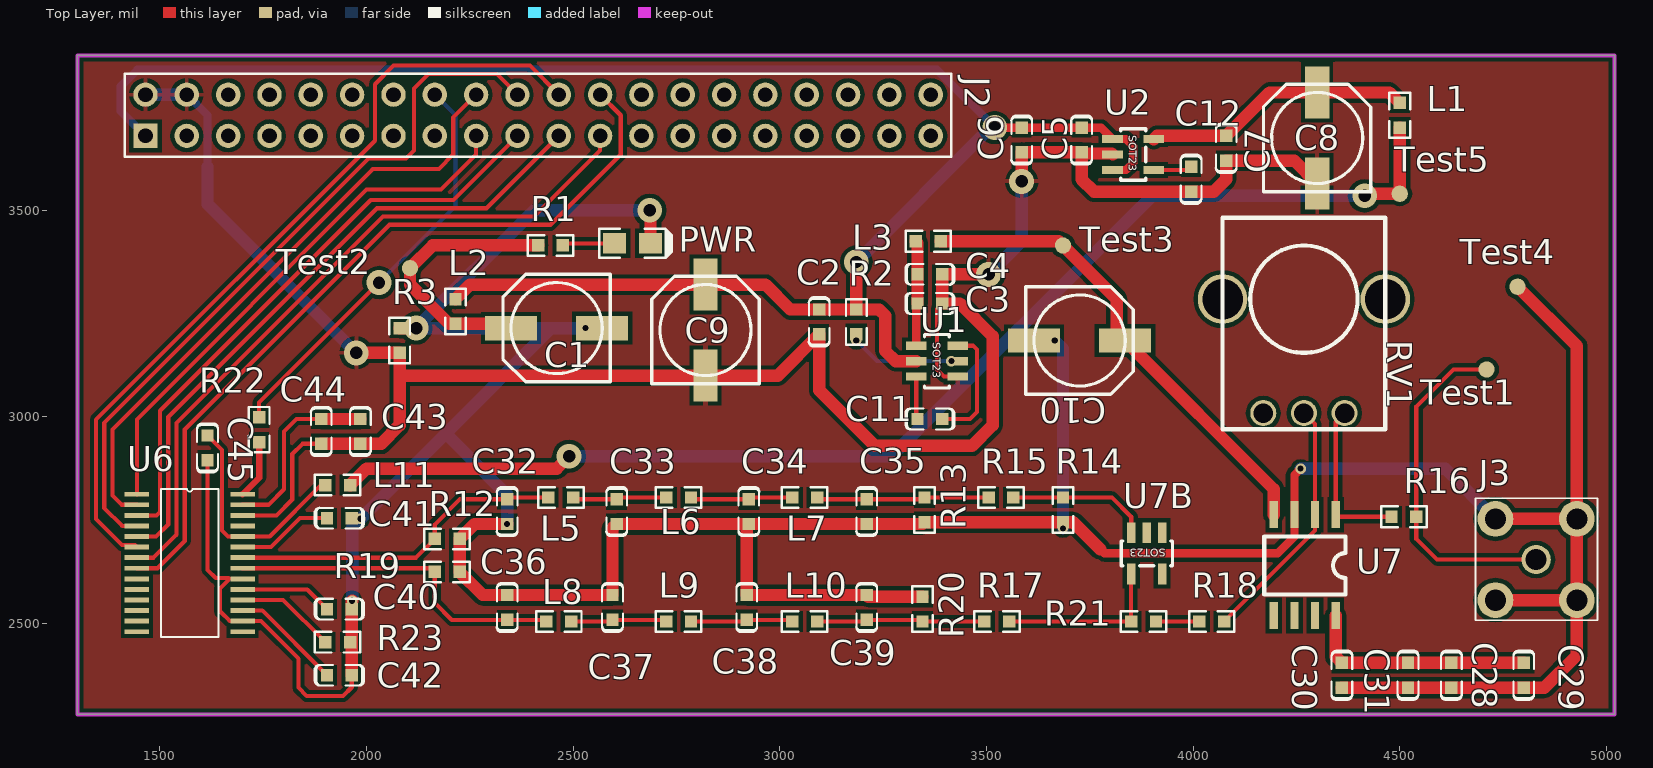
[diagram p0: Top Layer view]
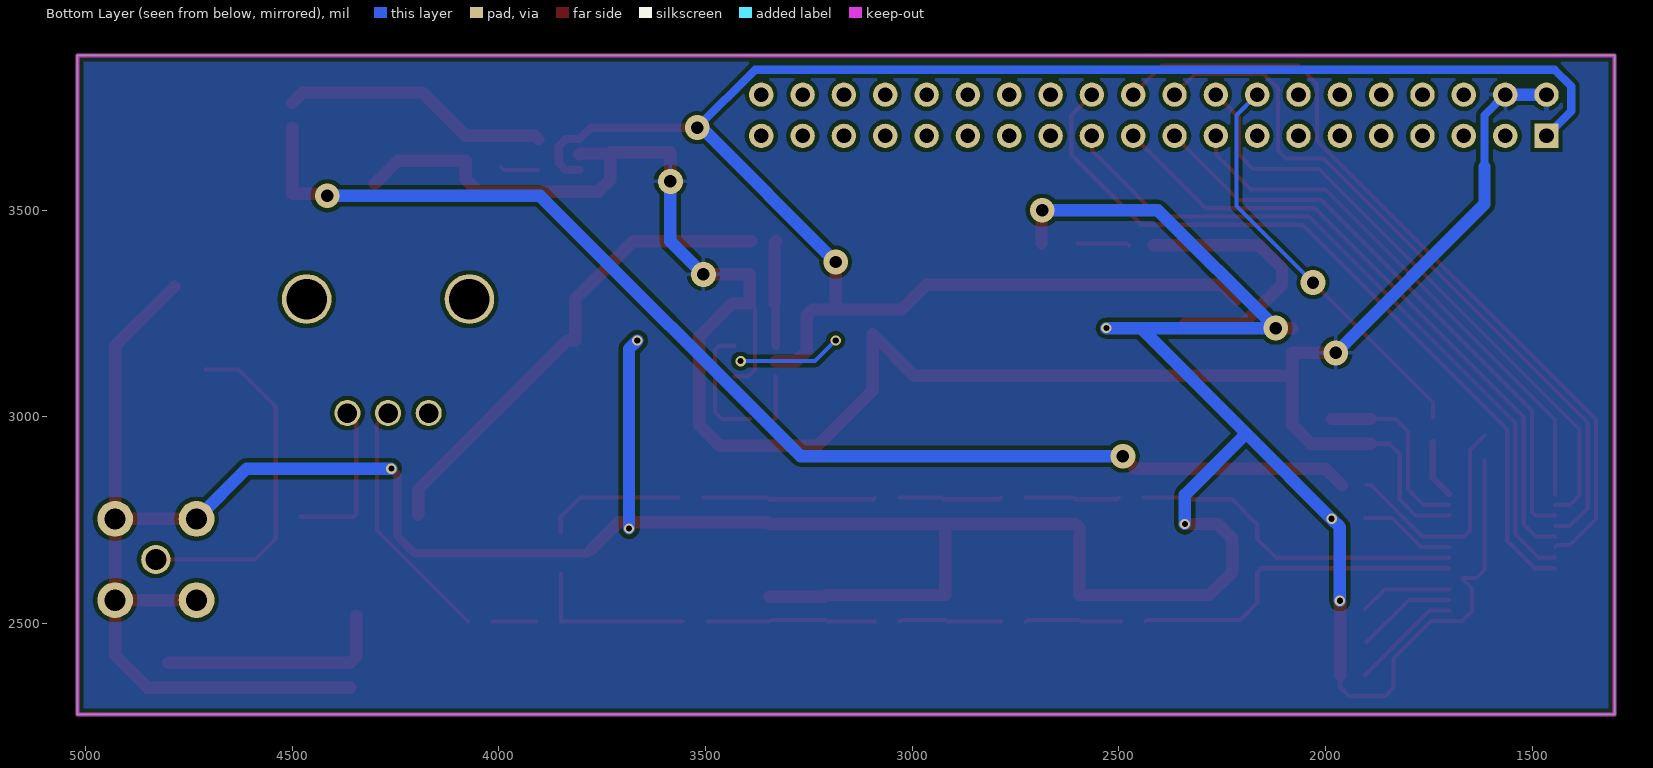
[diagram p1: Bottom Layer view, seen from below]
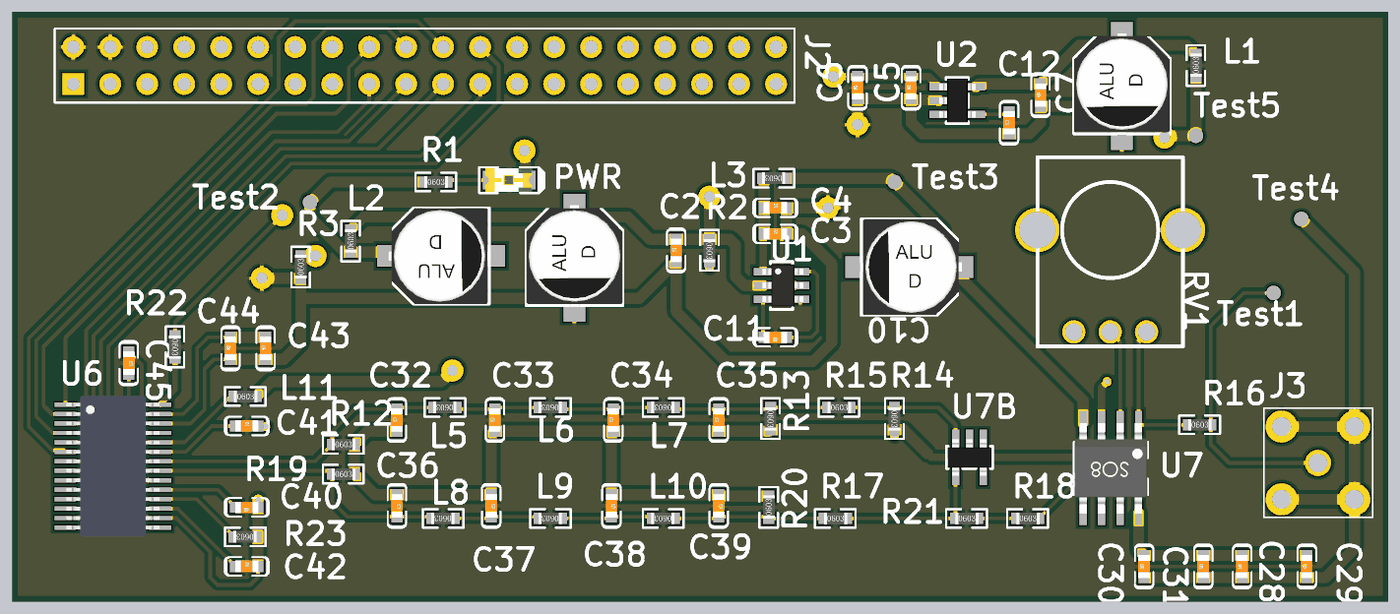
[diagram p2: 3D render of the assembled board from above, using the file's embedded part models]
# Altium PCB MISC68235.PcbDoc
Units mil, origin at the board's own origin, x right, y up, seen from the top; angles counter-clockwise.
Board outline 3720 x 1595 mil, 2 copper layers (Top Layer, Bottom Layer); 69 components, 44 nets, 219 pads, 19 vias.

## Layer stack, top to bottom (the 12.6 mil dielectric is the usual default, probably not edited)
Top Solder: solder mask 0.4, Solder Resist, Dk 3.5
Top Layer: signal copper 1.4
Dielectric 1: dielectric 12.6, FR-4, Dk 4.8
Bottom Layer: signal copper 1.4
Bottom Solder: solder mask 0.4, Solder Resist, Dk 3.5

## Board outline
1300,2280 5020,2280 5020,3875 1300,3875

## Design rules (kind name [scope] priority, off if disabled: settings)
Clearance [All] p1: gap=10 ignorepadtopadclearanceinfootprint=FALSE except(0: Arc-Hole Track-Hole SMDPad-Hole THPad-Hole Via-Hole Fill-Hole Poly-Hole Region-Hole Text-Hole)
MinimumSolderMaskSliver [All] p1: minsoldermaskwidth=0
PolygonConnect [All] p1: connectstyle=Relief reliefconductorwidth=10 reliefentries=4 polygonreliefangle="90 Angle" airgapwidth=10
RoutingVias [All] p1: holewidth=28 width=50 viastyle="Through Hole" minholewidth=28 minwidth=50 maxholewidth=28 maxwidth=50
SilkToSilkClearance [All] p1: silktosilkclearance=0
SilkToSolderMaskClearance [IsPad] p1: minsilkscreentomaskgap=0 clearancetoexposedcopper=TRUE
SolderMaskExpansion [All] p1: expansion=4
Width [All] p1: maxlimit=30 minlimit=10 preferedwidth=10
27 further rules are at their usual default settings.

## Components (designator, comment, footprint, x,y, rotation, side; value= is the part's Value field where it differs from the comment)
C1 "470uF/10V" "CS 6.3mm*5.4mm" 2349.76,3215 r0 top
C2 "3.3uF" CAP-SMD-0603 3095,3200 r90 top
C3 "3.3uF" CAP-SMD-0603 3333.03,3274.41 r0 top
C4 "10uF" CAP-SMD-0603 3333.03,3345 r0 top
C5 "10uF" CAP-SMD-0603 3730,3640 r90 top
C6 "104" CAP-SMD-0603 3585,3640 r90 top
C7 "104" CAP-SMD-0603 4080,3620 r90 top
C8 "470uF/10V" "CS 6.3mm*5.4mm" 4300,3785 r270 top
C9 "470uF/10V" "CS 6.3mm*5.4mm" 2820,3320.24 r270 top
C10 "4700uF/10V" "CS 6.3mm*5.4mm" 3835.24,3185 r180 top
C11 "3.3uF" CAP-SMD-0603 3393.03,2995 r180 top
C12 "233" CAP-SMD-0603 3995,3545 r90 top
C28 "10uF" CAP-SMD-0603 4625,2345 r90 top
C29 "104" CAP-SMD-0603 4800,2345 r90 top
C30 "10uF" CAP-SMD-0603 4360,2345 r90 top
C31 "104" CAP-SMD-0603 4520,2345 r90 top
C32 "100pF" CAP-SMD-0603 2340,2740.97 r90 top
C33 "NF" CAP-SMD-0603 2605,2740.97 r90 top
C34 "NF" CAP-SMD-0603 2925,2740.97 r90 top
C35 "NF" CAP-SMD-0603 3210,2740.97 r90 top
C36 "100pF" CAP-SMD-0603 2340,2569.03 r270 top
C37 "NF" CAP-SMD-0603 2595,2569.03 r270 top
C38 "100pF" CAP-SMD-0603 2920,2569.03 r270 top
C39 "NF" CAP-SMD-0603 3210,2569.03 r270 top
C40 "104" CAP-SMD-0603 1964.03,2535 r180 top
C41 "104" CAP-SMD-0603 1904.03,2755 r0 top
C42 "104" CAP-SMD-0603 1904.03,2375 r0 top
C43 "104" CAP-SMD-0603 1985,2935 r90 top
C44 "1uF" CAP-SMD-0603 1890,2935 r90 top
C45 "104" CAP-SMD-0603 1615,2955 r270 top
J2 "Header-HS_AD_DA-2*20-2.54mm" HEADER-HS-AD-DA-2*20-2.54MM 1465,3680 r0 top
J3 "SMA-KWE" SMA-KHD 4928.43,2753.43 r180 top
L1 "22uH" RES-SMD-0603 4500,3700 r90 top
L2 "22uH" RES-SMD-0603 2215,3225 r90 top
L3 "22uH" RES-SMD-0603 3389,3425 r180 top
L5 "470nH" RES-SMD-0603 2500,2805 r180 top
L6 "820nH" RES-SMD-0603 2785,2805 r180 top
L7 "470nH" RES-SMD-0603 3090,2805 r180 top
L8 "470nH" RES-SMD-0603 2495,2505 r180 top
L9 "820nH" RES-SMD-0603 2785,2505 r180 top
L10 "470nH" RES-SMD-0603 3090,2505 r180 top
L11 "22uH" RES-SMD-0603 1900,2835 r0 top
PWR "LED-0805" LED-SMD-0805 2600,3420 r0 top
R1 "510R" RES-SMD-0603 2415,3415 r0 top
R2 "10K" RES-SMD-0603 3185,3260 r270 top
R3 "0R" RES-SMD-0603 2080,3155 r90 top
R12 "100R" RES-SMD-0603 2165,2705 r0 top
R13 "100R" RES-SMD-0603 3350,2805 r270 top
R14 "1K" RES-SMD-0603 3685,2805 r270 top
R15 "1K" RES-SMD-0603 3505,2805 r0 top
R16 "51R" RES-SMD-0603 4480,2758.43 r0 top
R17 "1K" RES-SMD-0603 3495,2505 r0 top
R18 "1K" RES-SMD-0603 4015,2505 r0 top
R19 "100R" RES-SMD-0603 2165,2625 r0 top
R20 "100R" RES-SMD-0603 3345,2505 r90 top
R21 "1K" RES-SMD-0603 3850,2505 r0 top
R22 "33R" RES-SMD-0603 1740,2999.03 r270 top
R23 "2K" RES-SMD-0603 1960,2455 r180 top
RV1 "10K" RES-RV09 4169.72,3009.41 r0 top
Test1 "Test" Test 4710,3115 r90 top
Test2 "Test" Test 2105,3360 r0 top
Test3 "Test" Test 3685,3415 r90 top
Test4 "Test" Test 4785,3315 r90 top
Test5 "Test" Test 4500,3540 r90 top
U1 "SGM3204" SOT-23-6 3330,3172.4 r0 top
U2 "RT9193-3.3" SOT-23-5 3805,3672.4 r0 top
U6 "3PD9708E" TSSOP-28-NoHot 1444.09,2812.95 r0 top
U7 "LMH6643" SOIC-8 4345,2763.54 r270 top
U7B "LMH6643" SOT-23-5 3925,2720 r270 top

## Footprints (in the part's own frame and the unit in brackets; to place one, negate y for a bottom-side part, rotate by r counter-clockwise, add the part's x,y. Pads: shape width x height; smd on the part's side, far side on the other; paste and mask are expansions set on the pad)
CAP-SMD-0603 [mil]
  rect 30x30 smd: 1(0,0) 2(60,0)
  silkscreen extent -30,-25 90,25, body extent -1,-15 61,16, height 12
"CS 6.3mm*5.4mm" [mm]
  rect 3.2x1.5 smd: 1(0,0) 2(5.594,0)
  silkscreen extent -0.51,-3.3 6.1,3.3, body extent -0.82,-3.3 6.18,3.3, height 5.4
HEADER-HS-AD-DA-2*20-2.54MM [mm]
  rect 1.5x1.5 hole 0.9: 1(0,0)
  round 1.5 hole 0.9: 2(0,2.54) 3(2.54,0) 4(2.54,2.54) 5(5.08,0) 6(5.08,2.54) 7(7.62,0) 8(7.62,2.54) 9(10.16,0) 10(10.16,2.54) 11(12.7,0) 12(12.7,2.54) 13(15.24,0) 14(15.24,2.54) 15(17.78,0) 16(17.78,2.54) 17(20.32,0) 18(20.32,2.54) 19(22.86,0) 20(22.86,2.54) 21(25.4,0) 22(25.4,2.54) 23(27.94,0) 24(27.94,2.54) 25(30.48,0) 26(30.48,2.54) 27(33.02,0) 28(33.02,2.54) 29(35.56,0) 30(35.56,2.54) 31(38.1,0) 32(38.1,2.54) 33(40.64,0) 34(40.64,2.54) 35(43.18,0) 36(43.18,2.54) 37(45.72,0) 38(45.72,2.54) 39(48.26,0) 40(48.26,2.54)
  silkscreen extent -1.27,-1.27 49.53,3.81
LED-SMD-0805 [mm]
  rect 1.4x1.27 smd: 1(0,0) 2(2.21,0)
  silkscreen extent -0.95,-0.89 3.53,0.89, body extent -0.53,-0.8 2.68,0.8, height 1
RES-RV09 [mm]
  round 3.048 hole 2.5: 0(-2.5,7) 0(7.5,7)
  round 1.6 hole 1.2: 1(0,0) 2(2.5,0) 3(5,0)
  silkscreen extent -2.5,-1 7.5,12
RES-SMD-0603 [mil]
  rect 30x30 smd: 1(0,0) 2(60,0)
  silkscreen extent -25,-25 85,25, body extent 0,-16 62,15, height 18
SMA-KHD [mm]
  round 1.8 hole 1.3: 1(2.5,2.5)
  round 2.2 hole 1.3: 2(0,0) 3(5,0) 4(5,5) 5(0,5)
  silkscreen extent -1.27,-1.27 6.23,6.23
SOIC-8 [mm]
  rect 1.65x0.5 smd: 1(0,0) 2(0,-1.27) 3(0,-2.54) 4(0,-3.81) 5(6.2,-3.81) 6(6.2,-2.54) 7(6.2,-1.27) 8(6.2,0)
  silkscreen extent 1.35,-4.39 4.9,0.59, body extent 0.02,-4.41 6.22,0.59, height 1.75
SOT-23-5 [mil]
  rect 50x20 smd: 1(0,0) 2(0,-37.4) 3(0,-74.8) 4(100,-74.8) 5(100,0)
  silkscreen extent 20,-99 80,25, body extent 1,-96 99,22, height 41
SOT-23-6 [mil]
  rect 50x20 smd: 1(0,0) 2(0,-37.4) 3(0,-74.8) 4(100,-74.8) 5(100,-37.4) 6(100,0)
  silkscreen extent 20,-102 80,27, body extent -2,-94 108,20, height 57
Test [mm]
  round 1 smd: 1(0,0)
TSSOP-28-NoHot [mm]
  rect 1.5x0.3 smd: 1(0,0) 2(0,-0.65) 3(0,-1.3) 4(0,-1.95) 5(0,-2.6) 6(0,-3.25) 7(0,-3.9) 8(0,-4.55) 9(0,-5.2) 10(0,-5.85) 11(0,-6.5) 12(0,-7.15) 13(0,-7.8) 14(0,-8.45) 15(6.5,-8.45) 16(6.5,-7.8) 17(6.5,-7.15) 18(6.5,-6.5) 19(6.5,-5.85) 20(6.5,-5.2) 21(6.5,-4.55) 22(6.5,-3.9) 23(6.5,-3.25) 24(6.5,-2.6) 25(6.5,-1.95) 26(6.5,-1.3) 27(6.5,-0.65) 28(6.5,0)
  silkscreen extent 1.48,-8.78 5.02,0.33, body extent 0.05,-9.07 6.45,0.62, height 1.02

## Part data
C1 C8 C9 C10: library part C-CAP-SMD-220uF/10V
C2 C3 C4 C5 C6 C7 C11 C12 C28 C29 C30 C31 C32 C33 C34 C35 C36 C37 C38 C39 C40 C41 C42 C43 C44 C45: library part C-0603-SMD
J2: "High-speed AD/DA module interface"
L1 L2 L3 L5 L6 L7 L8 L9 L10 L11: library part L-0603-SMD, "SMD inductor"
PWR: "LED"
R1 R2 R3 R12 R13 R14 R15 R16 R17 R18 R19 R20 R21 R22 R23: library part R-0603-SMD, "SMD resistor"
RV1: library part R-RV09, "RV09 adjustable potentiometer"
Test1 Test2 Test3 Test4 Test5: "Test point"
U1: library part U-SGM3204, "LDO, negative output, 200mA"
U6: library part U-AD9708, "High-speed DAC, 8bit/125MSPS"
U7: library part U-AD8066, "High-speed op amp, 145MHz, 2CH"
U7B: library part U-AD8065, "High-speed op amp, 145MHz, 1CH"

## Via types
v1: diameter 60, hole 30, Top Layer to Bottom Layer, 10 vias
v2: diameter 25, hole 15, Top Layer to Bottom Layer, 9 vias

## Nets (pads, with @x,y where several pads share a name; then routed paths per layer and width w, separated by ;. In a path a pad name is that pad's centre, name@x,y a point inside that pad or via, vN(x,y) a via of type N, cw(c..) or ccw(c..) an arc to the next point about the centre after c; other vN are vias at no path point)
AGND: C1.2 C10.2 C28.1 C29.1 C30.1 C31.1 C32.1 C33.1 C34.1 C35.1 C36.1 C37.1 C38.1 C39.1 C40.1 C41.2 C42.2 C45.2 J3.2 J3.3 J3.4 J3.5 PWR.2 R3.2 R12.2 R13.2 R14.2 R19.2 R20.2 R23.1 Test4.1 U6.16 U6.20 U7.3 | length 9603.1
  Top Layer w10: C45.2 1615,2630 1635,2610 1666.46,2610 1668.23,2608.23 1645,2585 1645,2529.81 1668.94,2505.87 U6.16 1744.13,2505.87 1835,2415 1835,2345 1855,2325 1943.06,2325 1964.03,2345.97 C42.2
  Top Layer w20: 3775,2680 3785,2670 4204.64,2670 4245,2710.36 U7.3 4245,2860 v2(4260,2875)
  Top Layer w30: C42.2 1964.03,2554.03 v2(1965,2555) ; R3.2 v1(2120,3215) ; v2(2340,2740.97) 2260.97,2740.97 R12.2 R19.2 2280.97,2569.03 C36.1 C37.1 2595,2730.97 C33.1 C34.1 ; v1(2685,3500) 2687.01,3497.99 PWR.2 ; R20.2 3214.03,2565 C39.1 C38.1 2920,2735.97 C34.1 ; 3775,2680 3710,2745 R14.2 R13.2 3345.97,2740.97 C35.1 C34.1 ; C30.1 C31.1 C28.1 C29.1 4850,2345 4928.43,2423.43 J3.5 ; J3.4 J3.5 ; J3.3 J3.2 ; Test4.1 4928.43,3171.57 J3.2 ; J3.5 J3.2
  Bottom Layer w30: v2(1965,2555) 1965,2733.43 v2(1985,2753.43) 2191.57,2960 ; v2(2340,2740.97) 2340,2811.57 2191.57,2960 ; v2(2530,3215) 2446.57,3215 ; v1(2685,3500) 2405,3500 v1(2120,3215) 2446.57,3215 ; v2(3665,3185) 3685,3165 v2(3685,2730) ; v2(4260,2875) 4610,2875 J3.3 ; 2191.57,2960 2446.57,3215
AVCC_3V3: L1.1 L11.2 Test5.1 | length 2992
  Top Layer w30: L11.2 2000,2875 2460,2875 v1(2490,2905) ; v1(4415,3535) 4420,3540 Test5.1 L1.1
  Bottom Layer w30: v1(2490,2905) 3270,2905 3900,3535 v1(4415,3535)
D3V3: C43.2 C44.2 U6.27 | length 453
  Top Layer w10: U6.27 1762.36,2787.36 1800,2825 1800,2965 1830,2995 C44.2
  Top Layer w30: C44.2 C43.2
DA_CLK: J2.16 R22.1 | length 998.4
  Top Layer w10: R22.1 1740,3035 v1(2030,3325)
  Bottom Layer w10: v1(2030,3325) 2215,3510 2215,3730 J2.16
DA_D0: J2.24 U6.8 | length 1909.5
  Top Layer w10: U6.8 1493.82,2633.82 1560,2700 1560,2970 2055,3465 2445,3465 2615,3635 2615,3730 J2.24
DA_D1: J2.23 U6.7 | length 1722.4
  Top Layer w10: U6.7 1484.41,2659.41 1540,2715 1540,2985.15 2039.85,3485 2405,3485 2565,3645 J2.23
DA_D2: J2.22 U6.6 | length 1951.5
  Top Layer w10: U6.6 1439.41,2689.69 1408.35,2689.69 1345,2753.04 1345,2993.28 2020,3668.28 2020,3805 2065,3850 2395,3850 J2.22
DA_D3: J2.21 U6.5 | length 1574.8
  Top Layer w10: U6.5 1490.59,2710.59 1520,2740 1520,3000 2025,3505 2290,3505 J2.21
DA_D4: J2.20 U6.4 | length 1760.8
  Top Layer w10: U6.4 1408.82,2736.18 1365,2780 1365,2985 2005,3625 2095,3625 2115,3645 2115,3795 2150,3830 2315,3830 J2.20
DA_D5: J2.19 U6.3 | length 1444.8
  Top Layer w10: U6.3 1491.77,2761.77 1500,2770 1500,3015 2010,3525 2210,3525 J2.19
DA_D6: J2.18 U6.2 | length 1496.7
  Top Layer w10: U6.2 1407.64,2787.36 1385,2810 1385,2970 2015,3600 2175,3600 2209.53,3634.53 2209.53,3724.53 J2.18
DA_D7: J2.17 U6.1 | length 1312.5
  Top Layer w10: U6.1 1444.09,2994.09 2000,3550 2180,3550 2265,3635 J2.17
DVCC_3V3: C7.2 C8.1 L1.2 U2.5 | length 652
  Top Layer w30: U2.5 3912.6,3680 C7.2 4185,3785 C8.1 4475,3785 L1.2
GND: C2.1 C3.2 C4.2 C5.1 C6.1 C7.1 C8.2 C9.2 C12.1 C43.1 C44.1 J2.2 J2.4 R3.1 U1.4 U2.2 U6.26 | length 5441.1
  Top Layer w10: U6.26 1781.77,2761.77 1820,2800 1820,2910 1845,2935 C44.1 ; C3.2 3380,3261.38 3380,3115 3397.4,3097.6 U1.4
  Top Layer w30: C44.1 C43.1 2035,2935 2080,2980 2080,3105 ; v1(1975,3155) R3.1 2080,3105 ; v1(3505,3345) C4.2 C3.2 3435.59,3274.41 3515,3195 3515,2980 3465,2930 3230,2930 3095,3065 C2.1 2995,3100 C9.2 2085,3100 2080,3105 ; v1(3585,3570) C6.1 ; C6.1@3595,3640 C5.1 C5.1@3730,3637.4 ; U2.2 3802.6,3637.4 C5.1@3730,3637.4 ; C8.2 4244.76,3620 C7.1 4080,3575 4050,3545 C12.1 3760,3545 3730,3575 C5.1@3730,3637.4
  Bottom Layer w20: J2.4 1615,3730 1615,3605
  Bottom Layer w30: J2.2 J2.4 ; 1615,3605 1615,3515 v1(1975,3155) ; v1(3505,3345) 3585,3425 v1(3585,3570)
NetC11_1: C11.1 U1.6 | length 292.7
  Top Layer w10: C11.1 3460,2995 3476.77,3011.77 3476.77,3163.23 3467.6,3172.4 U1.6
NetC11_2: C11.2 U1.3 | length 103.9
  Top Layer w10: U1.3 3330,2998.03 C11.2
NetC12_2: C12.2 U2.4 | length 93.1
  Top Layer w10: U2.4 3987.6,3597.6 C12.2
NetC32_2: C32.2 L5.2 R12.1 U6.22 | length 820.8
  Top Layer w10: U6.22 2119.41,2659.41 R12.1 2165,2740 2225.97,2800.97 C32.2 2344.03,2805 L5.2
NetC33_2: C33.2 L5.1 L6.2 | length 228.3
  Top Layer w10: L5.1 2504.03,2800.97 C33.2 2609.03,2805 L6.2
NetC34_2: C34.2 L6.1 L7.2 | length 248.3
  Top Layer w10: L6.1 2789.03,2800.97 C34.2 2929.03,2805 L7.2
NetC35_2: C35.2 L7.1 R13.1 R15.1 | length 418.3
  Top Layer w10: L7.1 3094.03,2800.97 C35.2 3345.97,2800.97 R13.1 R15.1
NetC36_2: C36.2 L8.2 R19.1 U6.21 | length 832.3
  Top Layer w10: U6.21 2156.18,2633.82 R19.1 2165,2550 2205.97,2509.03 C36.2 2430.97,2509.03 L8.2
NetC37_2: C37.2 L8.1 L9.2 | length 233.3
  Top Layer w10: L8.1 2590.97,2505 C37.2 2720.97,2509.03 L9.2
NetC38_2: C38.2 L9.1 L10.2 | length 248.3
  Top Layer w10: L9.1 2915.97,2505 C38.2 3025.97,2509.03 L10.2
NetC39_2: C39.2 L10.1 R17.1 R20.1 | length 408.3
  Top Layer w10: L10.1 3205.97,2505 C39.2 3340.97,2509.03 R20.1 R17.1
NetC40_2: C40.2 U6.19 | length 223.8
  Top Layer w10: U6.19 1856.39,2582.64 C40.2
NetC41_1: C41.1 U6.23 | length 233
  Top Layer w10: U6.23 1769.03,2685 1839.03,2755 C41.1
NetC42_1: C42.1 U6.17 | length 268.8
  Top Layer w10: U6.17 1747.57,2531.46 C42.1
NetC45_1: C45.1 L11.1 U6.24 | length 552
  Top Layer w10: C45.1 1650,2920 1650,2725 1664.41,2710.59 U6.24 1765.59,2710.59 1890,2835 L11.1
NetJ3_1: J3.1 R16.2 Test1.1 | length 838
  Top Layer w10: Test1.1 4630,3115 4540,3025 R16.2 4540,2705 4590,2655 J3.1
NetPWR_1: PWR.1 R1.2 | length 127.1
  Top Layer w10: R1.2 2480,3420 PWR.1
NetR2_2: R2.2 U1.5 | length 250.7
  Bottom Layer w10: v2(3185,3185) 3235,3135 v2(3415,3135)
NetR14_1: R14.1 R15.2 U7B.3 | length 342.9
  Top Layer w10: R15.2 R14.1 3803.54,2805 3850.2,2758.35 U7B.3
NetR16_1: R16.1 RV1.3 U7.1 | length 391.9
  Top Layer w10: RV1.3 4345,2987.83 U7.1 4350.12,2758.43 R16.1
NetR17_2: R17.2 R21.1 U7B.4 | length 410.1
  Top Layer w10: R17.2 R21.1 3850,2619.8 U7B.4
NetR18_1: R18.1 R21.2 | length 105
  Top Layer w10: R21.2 R18.1
NetR18_2: R18.2 RV1.2 U7.2 | length 606.7
  Top Layer w10: R18.2 4295,2725 U7.2 4295,2982.56 RV1.2
NetR22_2: R22.2 U6.28 | length 142.6
  Top Layer w15: U6.28 1740,2852.95 R22.2
NetR23_2: R23.2 U6.18 | length 242.3
  Top Layer w10: U6.18 1797.95,2557.05 R23.2
"VCC  5V": C28.2 C29.2 C30.2 C31.2 U7.8 | length 560.7
  Top Layer w30: U7.8 4345,2420 C30.2 C31.2 C28.2 C29.2
"VCC  -IN": C3.1 C4.1 L3.2 U1.1 | length 255.5
  Top Layer w20: U1.1 3330,3271.38 C3.1
  Top Layer w30: L3.2 3333.03,3420.97 C4.1 C3.1
VCC_5V: C1.1 L2.1 R1.1 Test2.1 | length 661
  Top Layer w30: C1.1 2339.76,3225 L2.1 2200,3225 2105,3320 Test2.1 2160,3415 R1.1
VCC_-5V: C10.1 L3.1 Test3.1 U7.4 | length 1174.6
  Top Layer w30: L3.1 3675,3425 Test3.1 3815,3285 3815,3185 3835,3185 4195,2825 U7.4
VCC_IN: C2.2 C5.2 C6.2 C9.1 J2.1 L2.2 R2.1 U1.2 U2.1 U2.3 | length 4616
  Top Layer w20: v1(3520,3700) C6.2 C5.2 3777.4,3700 U2.1 3837.6,3672.4 3855,3655 3855,3615 3837.6,3597.6 U2.3
  Top Layer w30: L2.2 2250.24,3320.24 C9.1 2964.76,3320.24 3025,3260 C2.2 R2.1 ; v1(3185,3375) R2.1 ; U1.2 3280,3135 3255,3160 3255,3245 3240,3260 R2.1
  Bottom Layer w20: J2.1 1405,3740 1405,3800 1445,3840 3380,3840 v1(3520,3700)
  Bottom Layer w30: v1(3185,3375) v1@3510,3700
pads on no net: J2.3 J2.5 J2.6 J2.7 J2.8 J2.9 J2.10 J2.11 J2.12 J2.13 J2.14 J2.15 J2.25 J2.26 J2.27 J2.28 J2.29 J2.30 J2.31 J2.32 J2.33 J2.34 J2.35 J2.36 J2.37 J2.38 J2.39 J2.40 RV1.0 RV1.1 U6.9 U6.10 U6.11 U6.12 U6.13 U6.14 U6.15 U6.25 U7.5 U7.6 U7.7 U7B.1 U7B.2 U7B.5

## Polygon pours and split planes (outlines as drawn)
GND on Top Layer "Top Layer-No Net" (solid, remove dead copper, pour order 0): 1165,3970 1235,4040 5050,4040 5050,2160 5085,2125 4980,2020 1145,2020
GND on Bottom Layer "Top Layer-No Net" (solid, remove dead copper, pour order 2): 1090,4035 5110,4035 5155,3990 5155,2170 1155,2170 1010,2025

## Keep-outs
Keep-Out Layer:
  lines w10: 1300,2280 1380,2280 4750,2280 5020,2280 5020,3875 1380,3875 1300,3875 1300,2280